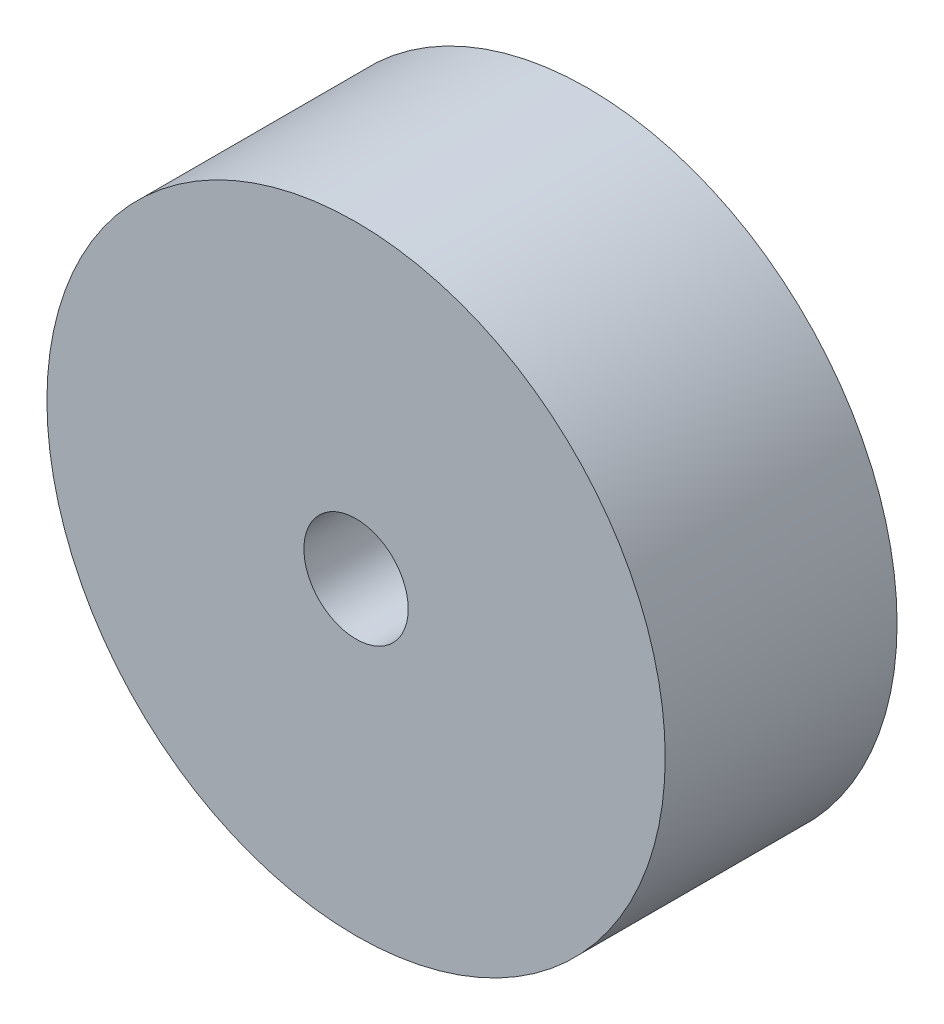
from build123d import *

# Parameters (mm, degrees)
SKETCH_1_R      = 24
SKETCH_1_R_2    = 4.05
EXTRUDE_1_DEPTH = 18


with BuildPart() as part:
    # 草图1 → 凸台-拉伸1 (new body)
    with BuildSketch(Plane.XY):
        Circle(SKETCH_1_R)
        Circle(SKETCH_1_R_2, mode=Mode.SUBTRACT)
    extrude(amount=EXTRUDE_1_DEPTH)


solid = part.part
